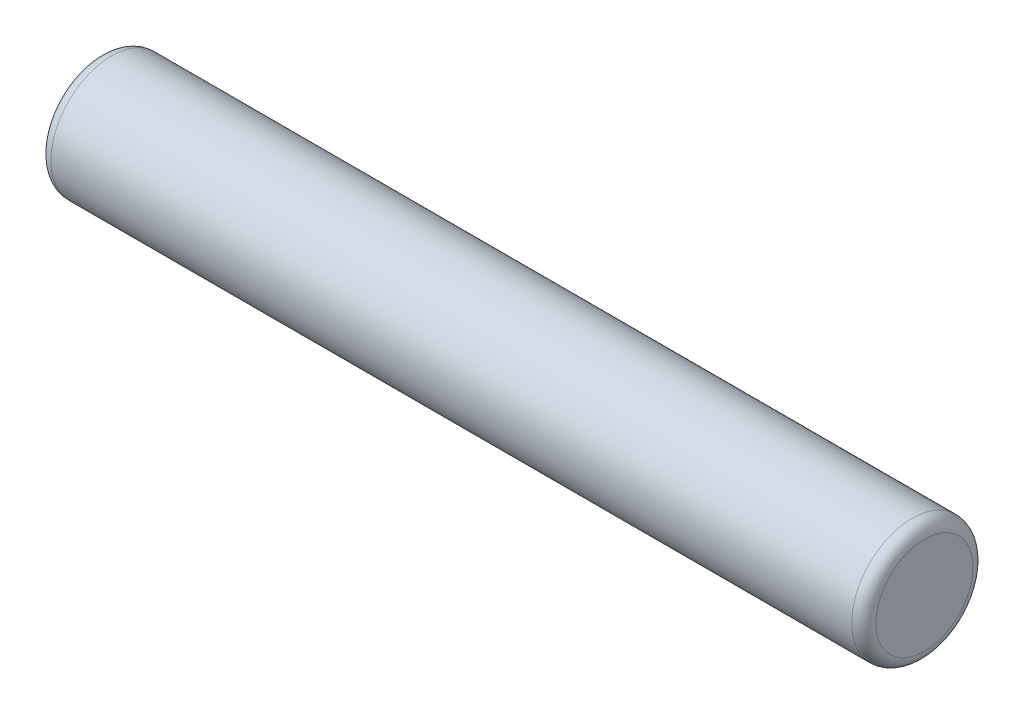
SolidWorks part; units mm, degrees
material "不锈钢304"
ref_plane "前视基准面" through (0, 0, 0) normal (0, 0, 1) x (1, 0, 0)
ref_plane "上视基准面" through (0, 0, 0) normal (0, 1, 0) x (1, 0, 0)
ref_plane "右视基准面" through (0, 0, 0) normal (1, 0, 0) x (0, 0, -1)
sketch "草图1" plane through (0, 0, 0) normal (1, 0, 0) x (0, 0, -1)
  circle A0 centre (0, 0) radius 1
  dimension "D1" = 2
extrude "凸台-拉伸1" add sketch "草图1" along normal mid plane 13.6
fillet "圆角1" radius 0.2 2 edges at (6.8, 0, -1) (-6.8, 0, -1)
